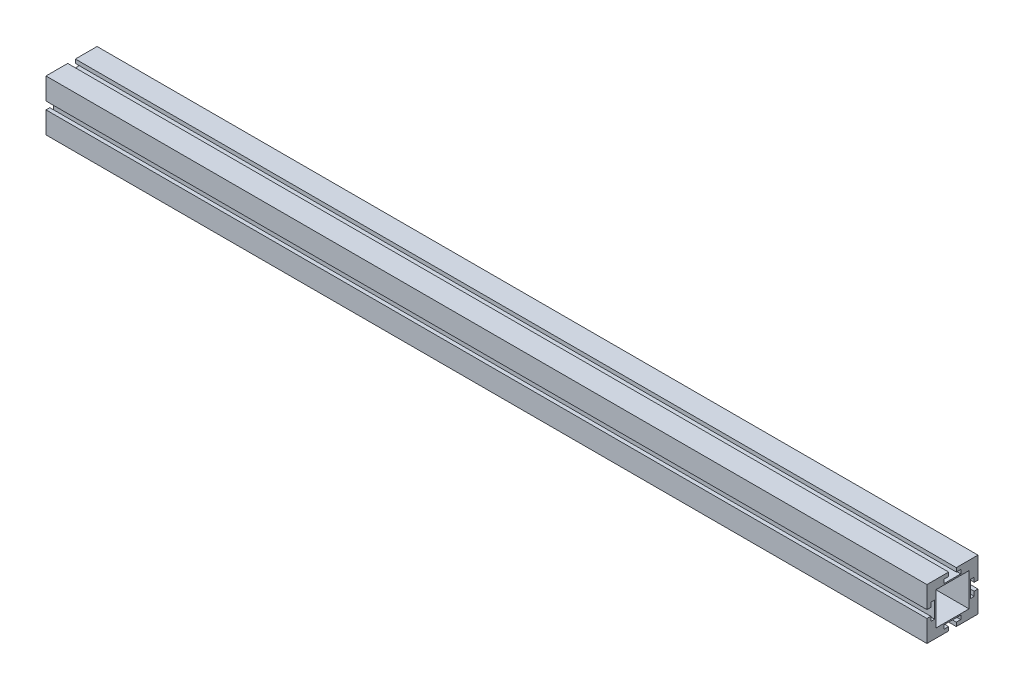
from build123d import *

# Parameters (mm, degrees)
SKETCH1_W           = 26
SKETCH1_H           = 26
BOSS_EXTRUDE1_DEPTH = 690


with BuildPart() as part:
    # Sketch1 → Boss-Extrude1 (new body)
    with BuildSketch(Plane(origin=(0, 0, 0), x_dir=(0, 0, -1), z_dir=(1, 0, 0))):
        Polygon((-20, -20), (-3, -20), (-3, -17), (-6.5, -17), (-6.5, -14), (6.5, -14), (6.5, -17), (3, -17), (3, -20), (20, -20), (20, -3), (17, -3), (17, -6.5), (14, -6.5), (14, 6.5), (17, 6.5), (17, 3), (20, 3), (20, 20), (3, 20), (3, 17), (6.5, 17), (6.5, 14), (-6.5, 14), (-6.5, 17), (-3, 17), (-3, 20), (-20, 20), (-20, 3), (-17, 3), (-17, 6.5), (-14, 6.5), (-14, -6.5), (-17, -6.5), (-17, -3), (-20, -3), align=None)
        Rectangle(SKETCH1_W, SKETCH1_H, mode=Mode.SUBTRACT)
    extrude(amount=BOSS_EXTRUDE1_DEPTH)


solid = part.part
